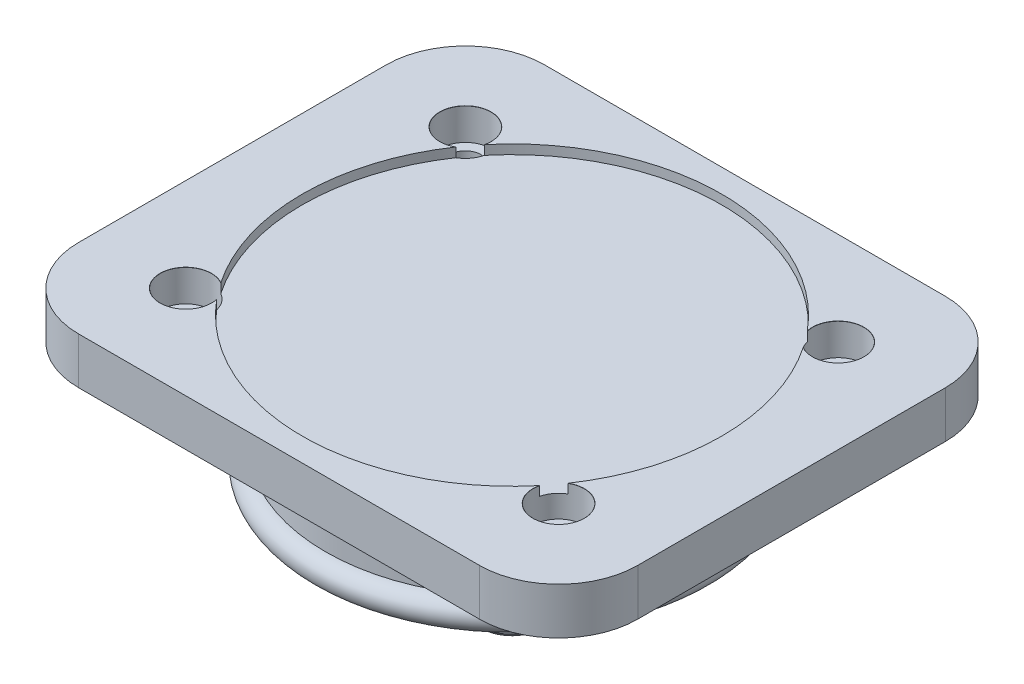
SolidWorks part; units mm, degrees
material "1050(GB)"
ref_plane "Front Plane" through (0, 0, 0) normal (0, 0, 1) x (1, 0, 0)
ref_plane "Top Plane" through (0, 0, 0) normal (0, 1, 0) x (1, 0, 0)
ref_plane "Right Plane" through (0, 0, 0) normal (1, 0, 0) x (0, 0, -1)
sketch "Sketch1" plane through (0, 0, 0) normal (0, 1, 0) x (1, 0, 0)
  line L0 (-60, 0) -> (60, 0) construction
  line L1 (-43, 50) -> (43, 50)
  line L2 (-60, 33) -> (-60, -33)
  line L3 (-43, -50) -> (43, -50)
  line L4 (60, 33) -> (60, -33)
  line L5 (-60, 50) -> (60, -50) construction
  line L6 (-60, -50) -> (60, 50) construction
  line L7 (0, 50) -> (0, -50) construction
  arc A0 (-60, 33) -> (-43, 50) centre (-43, 33) cw
  arc A1 (-60, -33) -> (-43, -50) centre (-43, -33) ccw
  arc A2 (43, -50) -> (60, -33) centre (43, -33) ccw
  arc A3 (60, 33) -> (43, 50) centre (43, 33) ccw
  point P0 (0, 0)
  dimension "D1" = 120
  dimension "D2" = 100
extrude "Boss-Extrude1" add sketch "Sketch1" along normal blind 10
sketch "Sketch2" plane through (0, 0, 0) normal (0, -1, 0) x (1, 0, 0)
  circle A0 centre (0, 0) radius 40
  dimension "D1" = 80
extrude "Boss-Extrude2" add sketch "Sketch2" along normal blind 20
sketch "Sketch3" plane through (0, 0, 0) normal (1, 0, 0) x (0, 0, -1)
  line L0 (-40, 0) -> (-40, -20) construction
  line L1 (0, 22.5152) -> (0, -31.5429) construction
  circle A0 centre (-40, -17) radius 3
  dimension "D1" = 6
revolve "Revolve1" add sketch "Sketch3" angle 360 about L1
sketch "Sketch4" plane through (0, -20, 0) normal (0, -1, 0) x (1, 0, 0)
  circle A0 centre (0, 0) radius 7.5
  dimension "D1" = 15
hole_wizard "CBORE for M6 Hexagon socket head cap screws1" positions "Sketch8" profile "Sketch9" counterbore size "M6" standard "GB" end condition through all
sketch "Sketch8" plane through (0, 10, 0) normal (0, 1, 0) x (1, 0, 0)
  line L0 (43, 50) -> (-43, 50) construction
  line L2 (60, -33) -> (60, 33) construction
  line L3 (-43, -50) -> (43, -50) construction
  line L4 (-60, 33) -> (-60, -33) construction
  point P0 (-40, 30)
  point P2 (40, 30)
  point P4 (40, -30)
  point P6 (-40, -30)
  dimension "D1" = 20
  dimension "D2" = 80
  dimension "D3" = 20
  dimension "D4" = 20
  dimension "D5" = 20
  dimension "D6" = 20
  dimension "D7" = 20
  dimension "D8" = 20
  dimension "D9" = 60
sketch "Sketch9" plane through (-40, 10, -30) normal (1, 0, 0) x (0, 0, 1)
  line L0 (0, 0) -> (0, 30)
  line L1 (0, 30) -> (3.3, 30)
  line L3 (3.3, 30) -> (3.3, 6.8)
  line L4 (5.5, 6.8) -> (3.3, 6.8)
  line L5 (5.5, 6.8) -> (5.5, 0.025)
  line L6 (5.5, 0.025) -> (5.525, 0)
  line L7 (5.525, 0) -> (0, 0)
  line L8 (-5.5, 0.025) -> (-5.525, 0) construction
  line L11 (0, -6.35) -> (0, 107.95) construction
  dimension "通孔孔直径" = 6.6
  dimension "通孔孔深度" = 30
  dimension "柱形沉头孔直径" = 11
  dimension "柱形沉头孔深度" = 6.8
  dimension "近端锥形沉头孔直径" = 11.05
  dimension "近端锥形沉头孔角度" = 90
extrude "Boss-Extrude3" add sketch "Sketch4" along normal blind 25
cosmetic thread "Cosmetic Thread1" parameters "D2"=11.797
chamfer "Chamfer1" distance 1 angle 45 1 edges at (0, -45, -7.5)
sketch "Sketch5" plane through (0, 10, 0) normal (0, 1, 0) x (1, 0, 0)
  circle A0 centre (0, 0) radius 45
  dimension "D1" = 90
extrude "Cut-Extrude1" cut sketch "Sketch5" against normal blind 2
